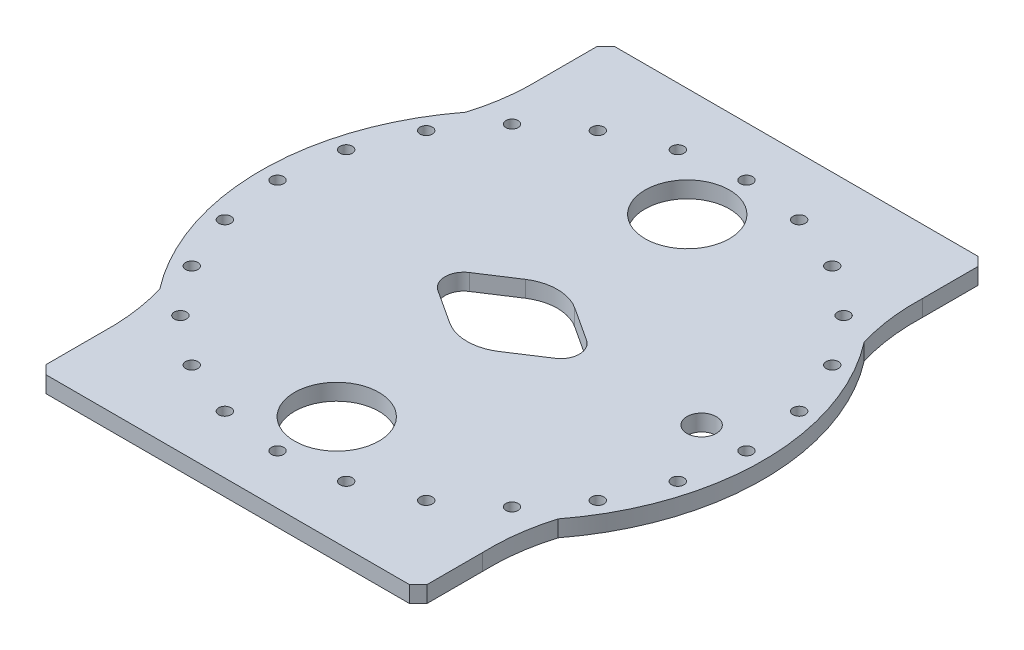
from build123d import *

# Parameters (mm, degrees)
SKETCH3_R           = 25
SKETCH3_R_2         = 72
BOSS_EXTRUDE1_DEPTH = 28
SKETCH4_R           = 10.5
CUT_EXTRUDE1_DEPTH  = 3671.216984417


with BuildPart() as part:
    # Sketch3 → Boss-Extrude1 (new body)
    with BuildSketch(Plane(origin=(0, 0, 0), x_dir=(1, 0, 0), z_dir=(0, 1, 0))):
        with BuildLine():
            Line((2845.680118699, 2169.501165066), (2845.680118699, 2074.501165066))
            ThreePointArc((2845.680118699, 2074.501165066), (2848.414414178, 2016.917733414), (2860.484776028, 1960.547223948))
            ThreePointArc((2860.484776028, 1960.547223948), (2949.180118699, 1699.501165066), (2860.484776028, 1438.455106185))
            ThreePointArc((2860.484776028, 1438.455106185), (2848.414414178, 1382.084596719), (2845.680118699, 1324.501165066))
            Line((2845.680118699, 1324.501165066), (2845.680118699, 1229.501165066))
            Line((2845.680118699, 1229.501165066), (2830.680118699, 1214.501165066))
            Line((2830.680118699, 1214.501165066), (2210.680118699, 1214.501165066))
            Line((2210.680118699, 1214.501165066), (2195.680118699, 1229.501165066))
            Line((2195.680118699, 1229.501165066), (2195.680118699, 1324.501165066))
            ThreePointArc((2195.680118699, 1324.501165066), (2192.94582322, 1382.084596719), (2180.87546137, 1438.455106185))
            ThreePointArc((2180.87546137, 1438.455106185), (2092.180118699, 1699.501165066), (2180.87546137, 1960.547223948))
            ThreePointArc((2180.87546137, 1960.547223948), (2192.94582322, 2016.917733414), (2195.680118699, 2074.501165066))
            Line((2195.680118699, 2074.501165066), (2195.680118699, 2169.501165066))
            Line((2195.680118699, 2169.501165066), (2210.680118699, 2184.501165066))
            Line((2210.680118699, 2184.501165066), (2830.680118699, 2184.501165066))
            Line((2830.680118699, 2184.501165066), (2845.680118699, 2169.501165066))
        make_face()
        with Locations(Location((2844.180118699, 1699.501165066, 0), (0, 0, 270))):
            Circle(SKETCH3_R, mode=Mode.SUBTRACT)
        with Locations(Location((2520.680118699, 1400.501165066, 0), (0, 0, 270))):
            Circle(SKETCH3_R_2, mode=Mode.SUBTRACT)
        with Locations(Location((2520.680118699, 1998.501165066, 0), (0, 0, 270))):
            Circle(SKETCH3_R_2, mode=Mode.SUBTRACT)
        with BuildLine():
            Line((2620.554891012, 1673.06787727), (2562.676931085, 1635.306037562))
            ThreePointArc((2562.676931085, 1635.306037562), (2520.680118699, 1622.914580714), (2478.683306313, 1635.306037562))
            Line((2478.683306313, 1635.306037562), (2420.805346386, 1673.06787727))
            ThreePointArc((2420.805346386, 1673.06787727), (2406.139786968, 1699.889370895), (2420.805346386, 1726.71086452))
            Line((2420.805346386, 1726.71086452), (2478.683306313, 1764.472704228))
            ThreePointArc((2478.683306313, 1764.472704228), (2520.680118699, 1776.864161076), (2562.676931085, 1764.472704228))
            Line((2562.676931085, 1764.472704228), (2620.554891012, 1726.71086452))
            ThreePointArc((2620.554891012, 1726.71086452), (2635.220450429, 1699.889370895), (2620.554891012, 1673.06787727))
        make_face(mode=Mode.SUBTRACT)
    extrude(amount=BOSS_EXTRUDE1_DEPTH)

    # Sketch4 → Cut-Extrude1 (cut, through all)
    with BuildSketch(Plane(origin=(0, 28, 0), x_dir=(1, 0, 0), z_dir=(0, 1, 0))):
        with Locations(Location((2520.680118699, 2099.501165066, 0), (0, 0, 270))):
            Circle(SKETCH4_R)
        with Locations(Location((2624.20773674, 2085.871495582, 0), (0, 0, 270))):
            Circle(SKETCH4_R)
        with Locations(Location((2720.680118699, 2045.91132658, 0), (0, 0, 270))):
            Circle(SKETCH4_R)
        with Locations(Location((2803.522831173, 1982.343877541, 0), (0, 0, 270))):
            Circle(SKETCH4_R)
        with Locations(Location((2867.090280213, 1899.501165066, 0), (0, 0, 270))):
            Circle(SKETCH4_R)
        with Locations(Location((2907.050449214, 1803.028783107, 0), (0, 0, 270))):
            Circle(SKETCH4_R)
        with Locations(Location((2920.680118699, 1699.501165066, 0), (0, 0, 270))):
            Circle(SKETCH4_R)
        with Locations(Location((2907.050449214, 1595.973547025, 0), (0, 0, 270))):
            Circle(SKETCH4_R)
        with Locations(Location((2867.090280213, 1499.501165066, 0), (0, 0, 270))):
            Circle(SKETCH4_R)
        with Locations(Location((2803.522831173, 1416.658452592, 0), (0, 0, 270))):
            Circle(SKETCH4_R)
        with Locations(Location((2720.680118699, 1353.091003552, 0), (0, 0, 270))):
            Circle(SKETCH4_R)
        with Locations(Location((2624.20773674, 1313.130834551, 0), (0, 0, 270))):
            Circle(SKETCH4_R)
        with Locations(Location((2520.680118699, 1299.501165066, 0), (0, 0, 270))):
            Circle(SKETCH4_R)
        with Locations(Location((2417.152500658, 1313.130834551, 0), (0, 0, 270))):
            Circle(SKETCH4_R)
        with Locations(Location((2320.680118699, 1353.091003552, 0), (0, 0, 270))):
            Circle(SKETCH4_R)
        with Locations(Location((2237.837406224, 1416.658452592, 0), (0, 0, 270))):
            Circle(SKETCH4_R)
        with Locations(Location((2174.269957185, 1499.501165066, 0), (0, 0, 270))):
            Circle(SKETCH4_R)
        with Locations(Location((2134.309788183, 1595.973547025, 0), (0, 0, 270))):
            Circle(SKETCH4_R)
        with Locations(Location((2120.680118699, 1699.501165066, 0), (0, 0, 270))):
            Circle(SKETCH4_R)
        with Locations(Location((2134.309788183, 1803.028783107, 0), (0, 0, 270))):
            Circle(SKETCH4_R)
        with Locations(Location((2174.269957185, 1899.501165066, 0), (0, 0, 270))):
            Circle(SKETCH4_R)
        with Locations(Location((2237.837406224, 1982.343877541, 0), (0, 0, 270))):
            Circle(SKETCH4_R)
        with Locations(Location((2320.680118699, 2045.91132658, 0), (0, 0, 270))):
            Circle(SKETCH4_R)
        with Locations(Location((2417.152500658, 2085.871495582, 0), (0, 0, 270))):
            Circle(SKETCH4_R)
    extrude(amount=-CUT_EXTRUDE1_DEPTH, mode=Mode.SUBTRACT)


solid = part.part
